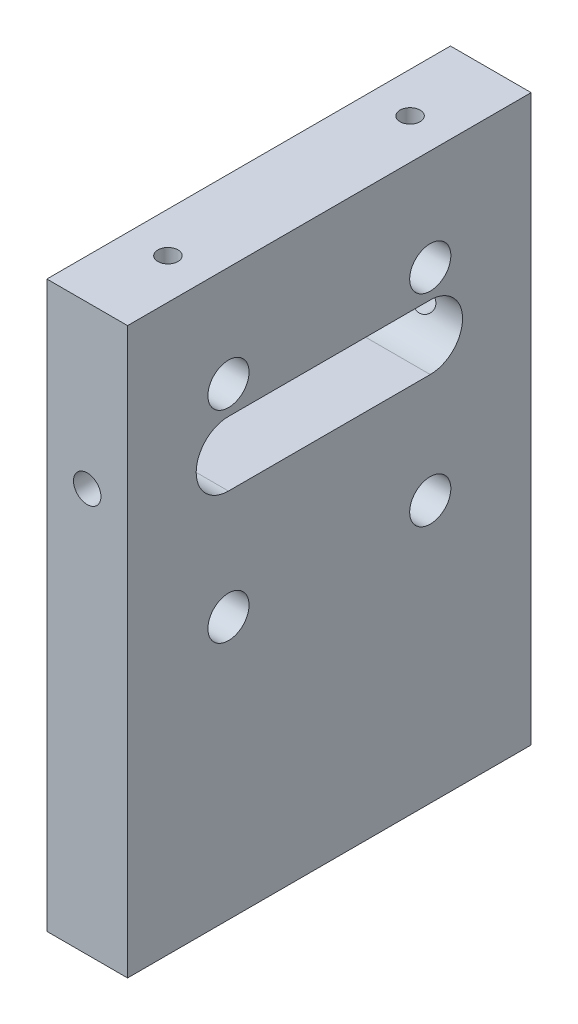
from build123d import *

# Parameters (mm, degrees)
SKETCH_1_W                    = 100
SKETCH_1_H                    = 140
EXTRUDE_1_DEPTH               = 20
HOLE_WIZARD_M6_1_D            = 5
HOLE_WIZARD_M6_1_DEPTH        = 15
HOLE_WIZARD_M6_1_TIP          = 1.502151548
CUT_EXTRUDE_1_DEPTH           = 89.317608663
HOLE_WIZARD_M8_1_D            = 6.8
HOLE_WIZARD_M12_1_D           = 10.2
HOLE_WIZARD_M12_1_CSINK_D     = 12.05
HOLE_WIZARD_M12_1_CSINK_ANGLE = 90
HOLE_WIZARD_M6_2_D            = 5
HOLE_WIZARD_M6_2_DEPTH        = 15
HOLE_WIZARD_M6_2_TIP          = 1.502151548


with BuildPart() as part:
    # 草图1 → 凸台-拉伸1 (new body)
    with BuildSketch(Plane(origin=(0, 0, 0), x_dir=(0, 0, -1), z_dir=(1, 0, 0))):
        Rectangle(SKETCH_1_W, SKETCH_1_H)
    extrude(amount=EXTRUDE_1_DEPTH)

    # M6 螺纹孔1
    with Locations(Plane(origin=(0, -70, 0), x_dir=(-1, 0, 0), z_dir=(0, -1, 0))):
        with Locations((-10, 30), (-10, -30)):
            Hole(HOLE_WIZARD_M6_1_D / 2, depth=HOLE_WIZARD_M6_1_DEPTH)
            with Locations((0, 0, -(HOLE_WIZARD_M6_1_DEPTH + HOLE_WIZARD_M6_1_TIP / 2))):  # 118° drill point
                Cone(0, HOLE_WIZARD_M6_1_D / 2, HOLE_WIZARD_M6_1_TIP, mode=Mode.SUBTRACT)

    # 草图4 → 切除-拉伸1 (cut, through all)
    with BuildSketch(Plane.ZY):
        with BuildLine():
            Line((-25, 38), (25, 38))
            ThreePointArc((25, 38), (33, 30), (25, 22))
            Line((25, 22), (-25, 22))
            ThreePointArc((-25, 22), (-33, 30), (-25, 38))
        make_face()
    extrude(amount=-CUT_EXTRUDE_1_DEPTH, mode=Mode.SUBTRACT)

    # M8 螺纹孔1 (through all)
    with Locations(Plane.XY.offset(50)):
        with Locations((10, 30)):
            Hole(HOLE_WIZARD_M8_1_D / 2)

    # M12 螺纹孔1 (through all)
    with Locations(Plane.ZY):
        with Locations((-25, 45), (25, 45), (-25, -5), (25, -5)):
            CounterSinkHole(HOLE_WIZARD_M12_1_D / 2, HOLE_WIZARD_M12_1_CSINK_D / 2, counter_sink_angle=HOLE_WIZARD_M12_1_CSINK_ANGLE)

    # M6 螺纹孔2
    with Locations(Plane(origin=(0, 70, 0), x_dir=(1, 0, 0), z_dir=(0, 1, 0))):
        with Locations((10, 30), (10, -30)):
            Hole(HOLE_WIZARD_M6_2_D / 2, depth=HOLE_WIZARD_M6_2_DEPTH)
            with Locations((0, 0, -(HOLE_WIZARD_M6_2_DEPTH + HOLE_WIZARD_M6_2_TIP / 2))):  # 118° drill point
                Cone(0, HOLE_WIZARD_M6_2_D / 2, HOLE_WIZARD_M6_2_TIP, mode=Mode.SUBTRACT)


solid = part.part
